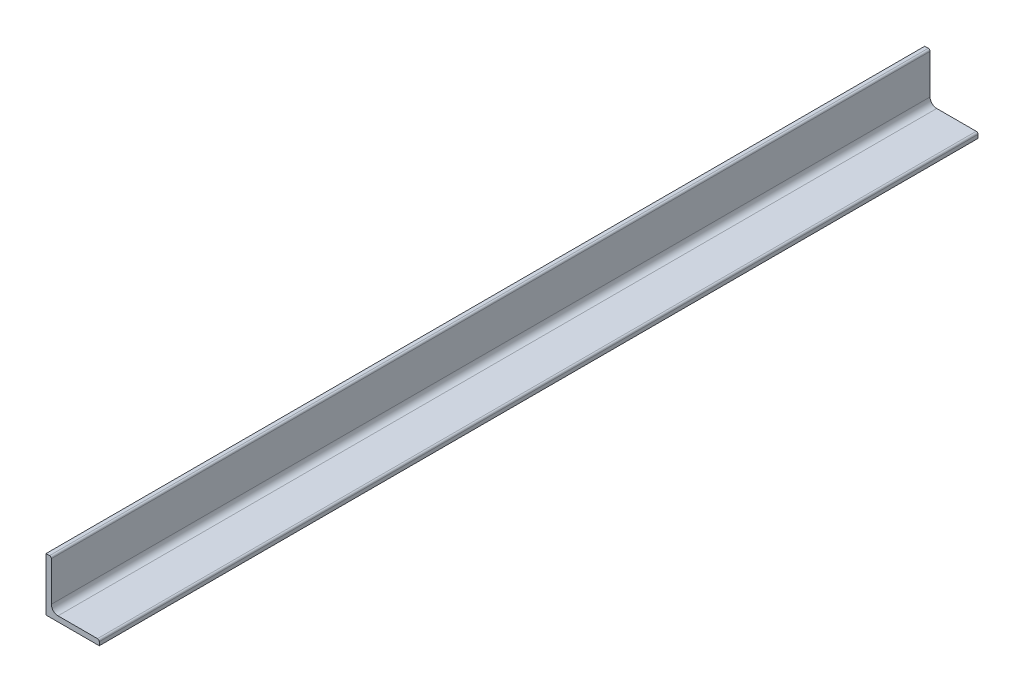
from build123d import *

# Parameters (mm, degrees)
BOSS_EXTRUDE1_DEPTH = 660


with BuildPart() as part:
    # Sketch1 → Boss-Extrude1 (new body)
    with BuildSketch(Plane.XY):
        with BuildLine():
            Line((0, 0), (0, 40))
            Line((0, 40), (2.666666667, 40))
            ThreePointArc((2.666666667, 40), (3.609475708, 39.609475708), (4, 38.666666667))
            Line((4, 38.666666667), (4, 9))
            ThreePointArc((4, 9), (5.464466094, 5.464466094), (9, 4))
            Line((9, 4), (38.666666667, 4))
            ThreePointArc((38.666666667, 4), (39.609475708, 3.609475708), (40, 2.666666667))
            Line((40, 2.666666667), (40, 0))
            Line((40, 0), (0, 0))
        make_face()
    extrude(amount=BOSS_EXTRUDE1_DEPTH)


solid = part.part
